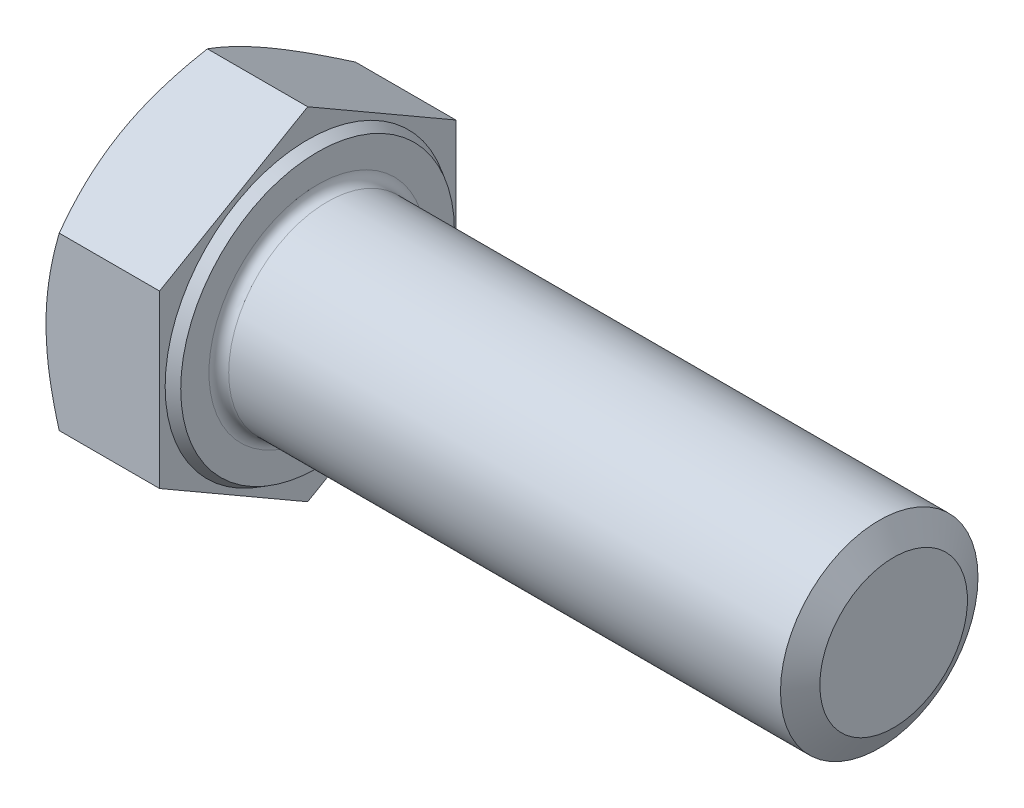
from build123d import *

# Parameters (mm, degrees)
EXTRUDE_393_DEPTH = 7.5
FILLET_1265_R     = 0.6


with BuildPart() as part:
    # 草图1 → Extrude 393 (new body)
    with BuildSketch(Plane(origin=(0, 0, 0), x_dir=(0, 0, -1), z_dir=(1, 0, 0))):
        Polygon((9, 5.196152423), (9, -5.196152423), (0, -10.392304845), (-9, -5.196152423), (-9, 5.196152423), (0, 10.392304845), align=None)
    extrude(amount=EXTRUDE_393_DEPTH)

    # 草图2 → 凸台-旋转1 (revolve)
    with BuildSketch(Plane.XY, mode=Mode.PRIVATE) as revolve_1_sk:
        Polygon((0, 0), (42.5, 0), (42.5, 4.4845), (42.5, 6), (0, 6), align=None)
    revolve(revolve_1_sk.sketch.rotate(Axis((0, 0, 0), (1, 0, 0)), 90), axis=Axis((0, 0, 0), (1, 0, 0)))

    # 草图3 → 切除-旋转1 (revolve, cut)
    with BuildSketch(Plane.XY):
        Polygon((0, 9), (3.690598923, 15.392304845), (3.690598923, 20.392304845), (-10, 20.392304845), (-10, 9), align=None)
    revolve(axis=Axis((0, 0, 0), (1, 0, 0)), mode=Mode.SUBTRACT)

    # 草图4 → 切除-旋转3 (revolve, cut)
    with BuildSketch(Plane.XY, mode=Mode.PRIVATE) as cut_revolve_3_sk:
        Polygon((7.5, 8.315), (6.9, 8.661410162), (6.9, 10.392304845), (7.5, 10.392304845), align=None)
    revolve(cut_revolve_3_sk.sketch.rotate(Axis((0, 0, 0), (1, 0, 0)), 90), axis=Axis((0, 0, 0), (1, 0, 0)), mode=Mode.SUBTRACT)

    # Fillet 1265
    fillet_1265_edges = [part.edges().sort_by_distance(p)[0] for p in [
        (7.5, 0, -6),
    ]]
    fillet(fillet_1265_edges, radius=FILLET_1265_R)

    # 草图6 → 切除-旋转4 (revolve, cut)
    with BuildSketch(Plane.XY, mode=Mode.PRIVATE) as cut_revolve_4_sk:
        Polygon((41.625, 6), (43.375, 6), (42.5, 4.484455543), align=None)
    revolve(cut_revolve_4_sk.sketch.rotate(Axis((0, 0, 0), (1, 0, 0)), 90), axis=Axis((0, 0, 0), (1, 0, 0)), mode=Mode.SUBTRACT)


solid = part.part
